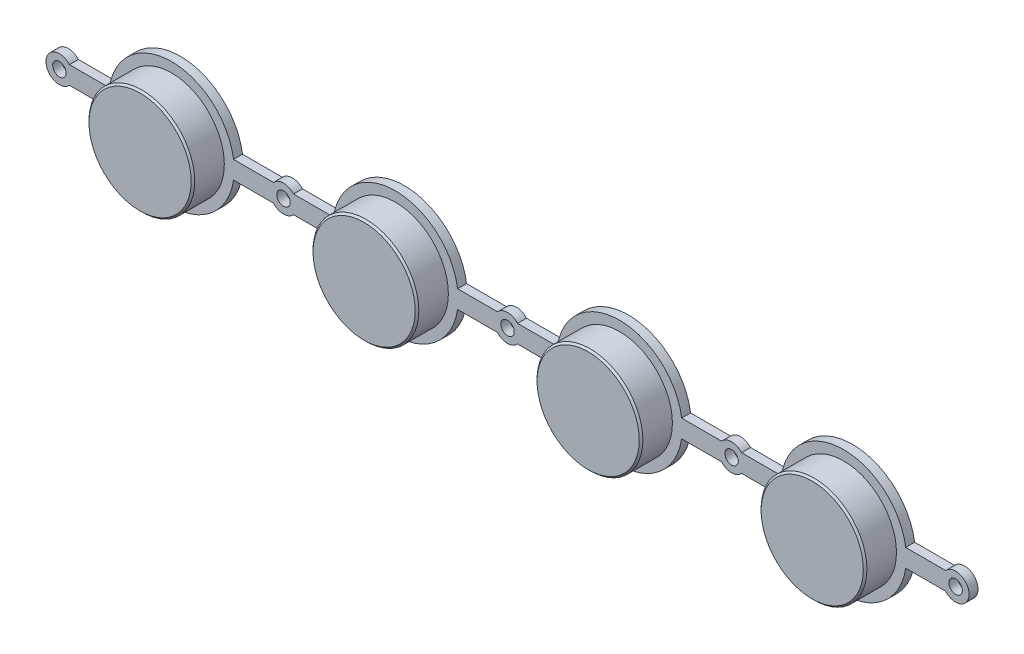
from build123d import *

# Parameters (mm, degrees)
SKETCH1_R           = 0.75
BOSS_EXTRUDE1_DEPTH = 1
SKETCH2_R           = 5.9
BOSS_EXTRUDE2_DEPTH = 3.5
CHAMFER1_SIZE       = 0.2
BOSS_EXTRUDE3_DEPTH = 2
CHAMFER2_SIZE       = 1.6


with BuildPart() as part:
    # Sketch1 → Boss-Extrude1 (new body)
    with BuildSketch(Plane.XY):
        with BuildLine():
            Line((-11.381966011, 1), (-6.92820323, 1))
            ThreePointArc((-6.92820323, 1), (0, 7), (6.92820323, 1))
            Line((6.92820323, 1), (11.381966011, 1))
            ThreePointArc((11.381966011, 1), (12.5, 1.5), (13.618033989, 1))
            Line((13.618033989, 1), (18.07179677, 1))
            ThreePointArc((18.07179677, 1), (25, 7), (31.92820323, 1))
            Line((31.92820323, 1), (36.381966011, 1))
            ThreePointArc((36.381966011, 1), (37.5, 1.5), (38.618033989, 1))
            Line((38.618033989, 1), (43.07179677, 1))
            ThreePointArc((43.07179677, 1), (50, 7), (56.92820323, 1))
            Line((56.92820323, 1), (61.381966011, 1))
            ThreePointArc((61.381966011, 1), (62.5, 1.5), (63.618033989, 1))
            Line((63.618033989, 1), (68.07179677, 1))
            ThreePointArc((68.07179677, 1), (75, 7), (81.92820323, 1))
            Line((81.92820323, 1), (86.381966011, 1))
            ThreePointArc((86.381966011, 1), (89, 0), (86.381966011, -1))
            Line((86.381966011, -1), (81.92820323, -1))
            ThreePointArc((81.92820323, -1), (75, -7), (68.07179677, -1))
            Line((68.07179677, -1), (63.618033989, -1))
            ThreePointArc((63.618033989, -1), (62.5, -1.5), (61.381966011, -1))
            Line((61.381966011, -1), (56.92820323, -1))
            ThreePointArc((56.92820323, -1), (50, -7), (43.07179677, -1))
            Line((43.07179677, -1), (38.618033989, -1))
            ThreePointArc((38.618033989, -1), (37.5, -1.5), (36.381966011, -1))
            Line((36.381966011, -1), (31.92820323, -1))
            ThreePointArc((31.92820323, -1), (25, -7), (18.07179677, -1))
            Line((18.07179677, -1), (13.618033989, -1))
            ThreePointArc((13.618033989, -1), (12.5, -1.5), (11.381966011, -1))
            Line((11.381966011, -1), (6.92820323, -1))
            ThreePointArc((6.92820323, -1), (0, -7), (-6.92820323, -1))
            Line((-6.92820323, -1), (-11.381966011, -1))
            ThreePointArc((-11.381966011, -1), (-14, 0), (-11.381966011, 1))
        make_face()
        with Locations((12.5, 0)):
            Circle(SKETCH1_R, mode=Mode.SUBTRACT)
        with Locations((37.5, 0)):
            Circle(SKETCH1_R, mode=Mode.SUBTRACT)
        with Locations((62.5, 0)):
            Circle(SKETCH1_R, mode=Mode.SUBTRACT)
        with Locations((-12.5, 0)):
            Circle(SKETCH1_R, mode=Mode.SUBTRACT)
        with Locations((87.5, 0)):
            Circle(SKETCH1_R, mode=Mode.SUBTRACT)
    extrude(amount=BOSS_EXTRUDE1_DEPTH)

    # Sketch2 → Boss-Extrude2 (add)
    with BuildSketch(Plane.XY.offset(1)):
        Circle(SKETCH2_R)
        with Locations((25, 0)):
            Circle(SKETCH2_R)
        with Locations((50, 0)):
            Circle(SKETCH2_R)
        with Locations((75, 0)):
            Circle(SKETCH2_R)
    extrude(amount=BOSS_EXTRUDE2_DEPTH)

    # Chamfer1
    chamfer1_edges = [part.edges().sort_by_distance(p)[0] for p in [
        (-5.9, 0, 4.5),
        (19.1, 0, 4.5),
        (44.1, 0, 4.5),
        (69.1, 0, 4.5),
    ]]
    chamfer(chamfer1_edges, length=CHAMFER1_SIZE)

    # Sketch3 → Boss-Extrude3 (add)
    with BuildSketch(Plane(origin=(0, 0, 0), x_dir=(-1, 0, 0), z_dir=(0, 0, -1))):
        Polygon((-74.25, -0.75), (-74.25, -4), (-75.75, -4), (-75.75, -0.75), (-79, -0.75), (-79, 0.75), (-75.75, 0.75), (-75.75, 4), (-74.25, 4), (-74.25, 0.75), (-71, 0.75), (-71, -0.75), align=None)
        Polygon((-50.75, 4), (-49.25, 4), (-49.25, 0.75), (-46, 0.75), (-46, -0.75), (-49.25, -0.75), (-49.25, -4), (-50.75, -4), (-50.75, -0.75), (-54, -0.75), (-54, 0.75), (-50.75, 0.75), align=None)
        Polygon((-29, 0.75), (-25.75, 0.75), (-25.75, 4), (-24.25, 4), (-24.25, 0.75), (-21, 0.75), (-21, -0.75), (-24.25, -0.75), (-24.25, -4), (-25.75, -4), (-25.75, -0.75), (-29, -0.75), align=None)
        Polygon((-4, 0.75), (-0.75, 0.75), (-0.75, 4), (0.75, 4), (0.75, 0.75), (4, 0.75), (4, -0.75), (0.75, -0.75), (0.75, -4), (-0.75, -4), (-0.75, -0.75), (-4, -0.75), align=None)
    extrude(amount=BOSS_EXTRUDE3_DEPTH)

    # Chamfer2
    chamfer2_edges = [part.edges().sort_by_distance(p)[0] for p in [
        (75, -4, -2),
        (71, 0, -2),
        (75, 4, -2),
        (79, 0, -2),
        (46, 0, -2),
        (50, 4, -2),
        (54, 0, -2),
        (50, -4, -2),
        (21, 0, -2),
        (25, 4, -2),
        (29, 0, -2),
        (25, -4, -2),
        (-4, 0, -2),
        (0, 4, -2),
        (4, 0, -2),
        (0, -4, -2),
    ]]
    chamfer(chamfer2_edges, length=CHAMFER2_SIZE)


solid = part.part
